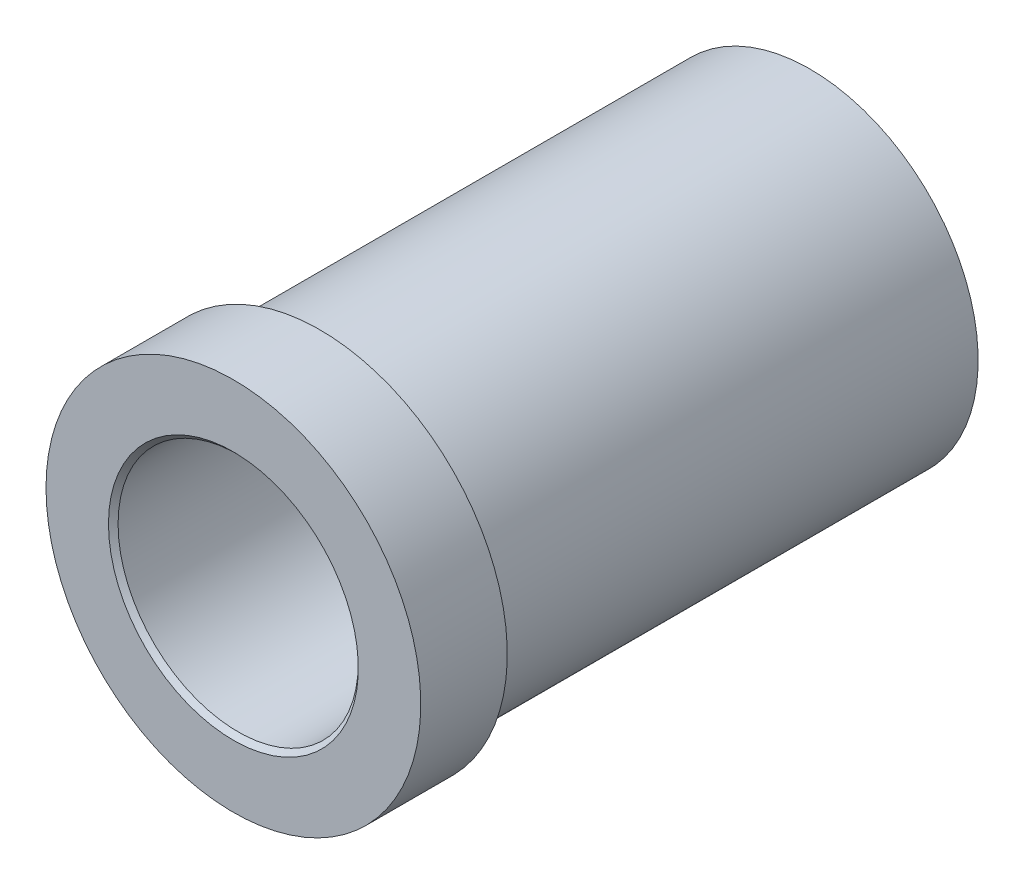
SolidWorks part; units mm, degrees
ref_plane "Front Plane" through (0, 0, 0) normal (0, 0, 1) x (1, 0, 0)
ref_plane "Top Plane" through (0, 0, 0) normal (0, 1, 0) x (1, 0, 0)
ref_plane "Right Plane" through (0, 0, 0) normal (1, 0, 0) x (0, 0, -1)
other "Configuration Table"
ref_plane "Plane1" through (0, 0, 0) normal (0, -1, 0) x (1, 0, 0)
sketch "Sketch1" plane through (0, 0, 0) normal (0, -1, 0) x (1, 0, 0)
  line L0 (19.5, 0) -> (19.5, 9)
  line L1 (19.5, 9) -> (13, 9)
  line L2 (13, 9) -> (12.5, 8.5)
  line L3 (12.5, 8.5) -> (12.5, -50.5)
  line L4 (12.5, -50.5) -> (13, -51)
  line L5 (13, -51) -> (17.5, -51)
  line L6 (17.5, -51) -> (17.5, 0)
  line L7 (17.5, 0) -> (19.5, 0)
  line L8 (0, 9) -> (0, -51) construction
  dimension "D1" = 12.5
  dimension "D2" = 13
  dimension "D3" = 17.5
  dimension "D4" = 19.5
  dimension "D5" = 0.5
  dimension "D6" = 51
  dimension "D7" = 59.5
  dimension "D8" = 60
revolve "Revolve1" add sketch "Sketch1" angle 360 about L8
